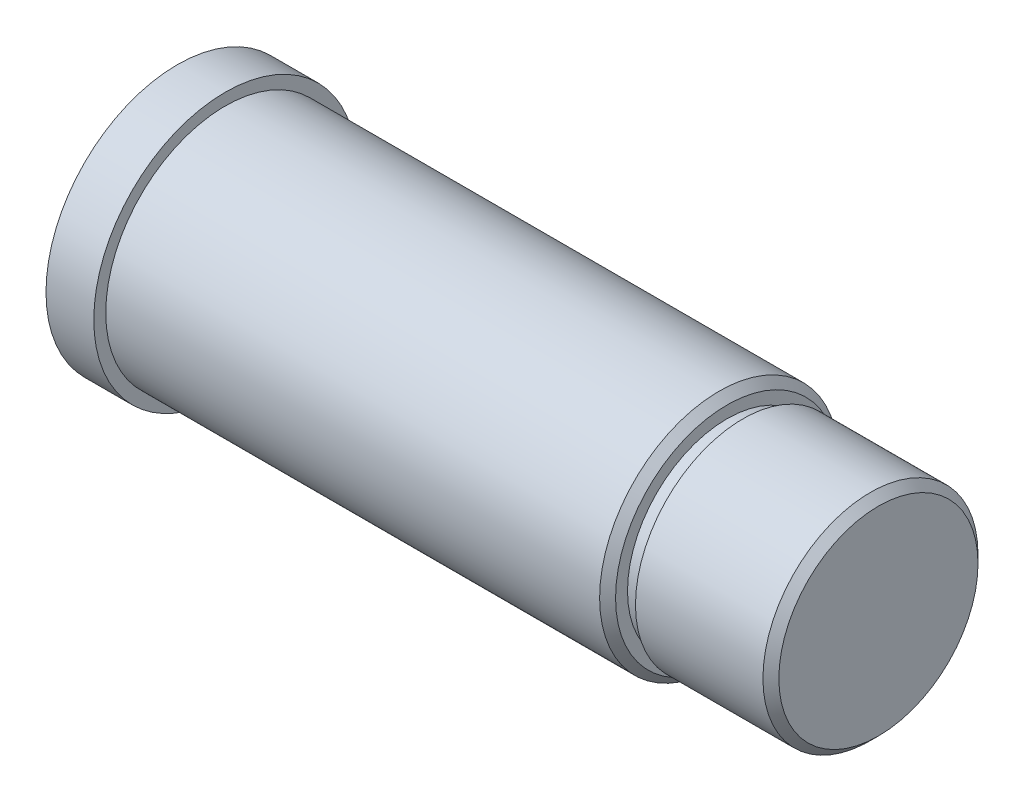
SolidWorks part; units mm, degrees
ref_plane "前视基准面" through (0, 0, 0) normal (0, 0, 1) x (1, 0, 0)
ref_plane "上视基准面" through (0, 0, 0) normal (0, 1, 0) x (1, 0, 0)
ref_plane "右视基准面" through (0, 0, 0) normal (1, 0, 0) x (0, 0, -1)
other "Configuration Table"
sketch "草图1" plane through (0, 0, 0) normal (0, 0, 1) x (1, 0, 0)
  line L0 (0, 0) -> (45.2635, 0) construction
  line L1 (0, 0) -> (0, 16.5)
  line L2 (0, 16.5) -> (6, 16.5)
  line L3 (6, 16.5) -> (6, 15)
  line L4 (6, 15) -> (69, 15)
  line L5 (69, 15) -> (69, 12.5)
  line L6 (69, 12.5) -> (71, 12.5)
  line L7 (71, 12.5) -> (71, 13.5)
  line L8 (71, 13.5) -> (88, 13.5)
  line L9 (88, 13.5) -> (88, 0)
  line L10 (0, 0) -> (88, 0)
  dimension "D1" = 16.5
  dimension "D2" = 15
  dimension "D3" = 12.5
  dimension "D4" = 13.5
  dimension "D5" = 6
  dimension "D6" = 63
  dimension "D7" = 2
  dimension "D8" = 88
revolve "旋转1" add sketch "草图1" angle 360 about L0
cosmetic thread "装饰螺纹线1" parameters "D2"=23.752
chamfer "倒角1" distance 1 angle 45 2 edges at (88, 0, 13.5) (69, 0, 15)
